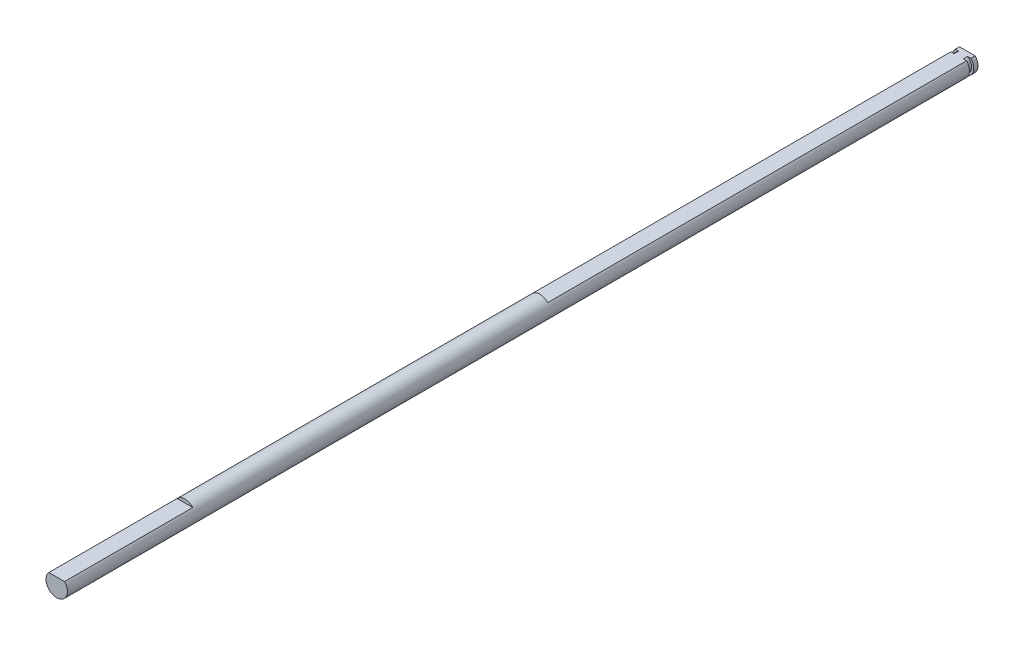
SolidWorks part; units mm, degrees
ref_plane "Front Plane" through (0, 0, 0) normal (0, 0, 1) x (1, 0, 0)
ref_plane "Top Plane" through (0, 0, 0) normal (0, 1, 0) x (1, 0, 0)
ref_plane "Right Plane" through (0, 0, 0) normal (1, 0, 0) x (0, 0, -1)
other "Configuration Table"
sketch "Sketch1" plane through (0, 0, 0) normal (0, 0, 1) x (1, 0, 0)
  circle A0 centre (0, 0) radius 2.5
  dimension "D1" = 5
extrude "Boss-Extrude1" add sketch "Sketch1" along normal blind 213
sketch "Sketch4" plane through (0, 0, 0) normal (0, 0, -1) x (-1, 0, 0)
  line L0 (0, 0) -> (0, 1.7) construction
  line L1 (-1.833, 1.7) -> (1.833, 1.7)
  circle A0 centre (0, 0) radius 2.5 construction
  arc A1 (1.833, 1.7) -> (-1.833, 1.7) centre (0, 0) ccw
  dimension "D1" = 1.7
extrude "Cut-Extrude2" cut sketch "Sketch4" against normal blind 100
ref_plane "Plane1" through (0, 0, 2) normal (0, 0, -1) x (-1, 0, 0)
sketch "Sketch5" plane through (0, 0, 2) normal (0, 0, -1) x (-1, 0, 0)
  circle A0 centre (0, 0) radius 2
  circle A1 centre (0, 0) radius 2.5
  dimension "D1" = 4
extrude "Cut-Extrude3" cut sketch "Sketch5" along normal blind 1
sketch "Sketch7" plane through (0, 0, 213) normal (0, 0, 1) x (1, 0, 0)
  line L0 (-1.835, 1.6979) -> (1.835, 1.6979)
  circle A0 centre (0, 0) radius 2.5 construction
  arc A1 (1.835, 1.6979) -> (-1.835, 1.6979) centre (0, 0) ccw
  dimension "D1" = 3.67
extrude "Cut-Extrude4" cut sketch "Sketch7" against normal blind 30
